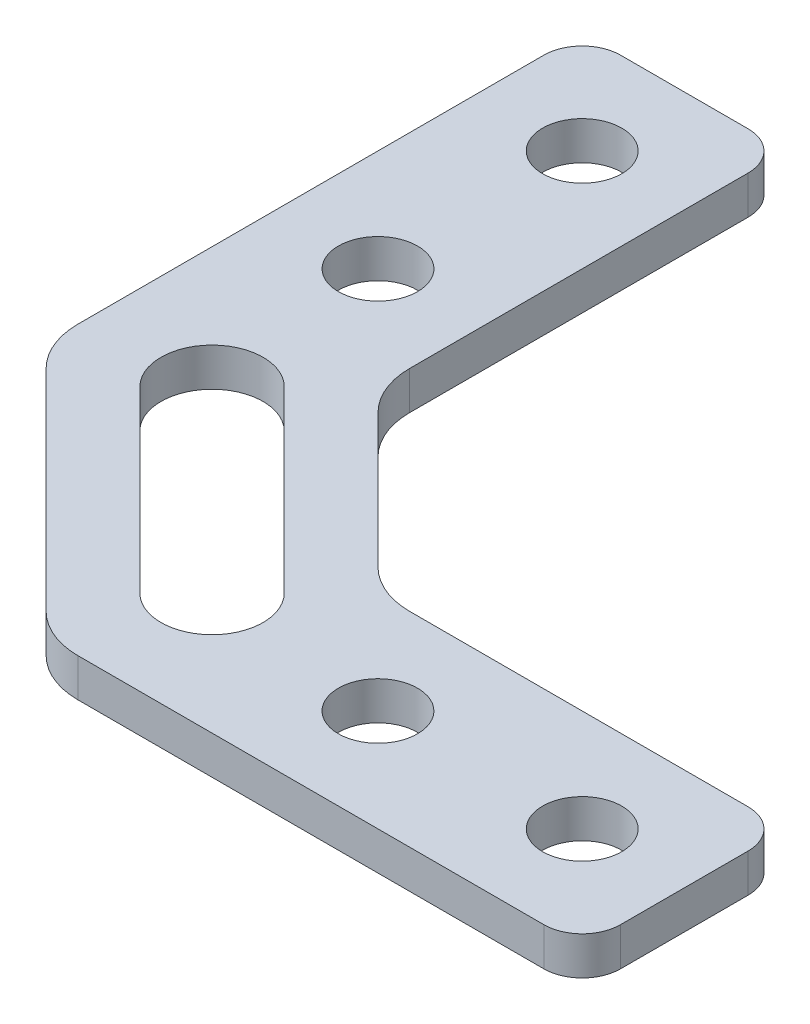
from build123d import *

# Parameters (mm, degrees)
SKETCH_1_R      = 1.55
EXTRUDE_1_DEPTH = 1.5
FILLET_1_R      = 1.5
FILLET_2_R      = 3


with BuildPart() as part:
    # 草图1 → 凸台-拉伸1 (new body)
    with BuildSketch(Plane(origin=(0, 0, 0), x_dir=(1, 0, 0), z_dir=(0, 1, 0))):
        Polygon((27, -4), (27, 4), (11, 4), (4, 11), (4, 27), (-4, 27), (-4, 6), (6, -4), align=None)
        with Locations(Location((15, 0, 0), (0, 0, 270))):
            Circle(SKETCH_1_R, mode=Mode.SUBTRACT)
        with Locations(Location((23, 0, 0), (0, 0, 270))):
            Circle(SKETCH_1_R, mode=Mode.SUBTRACT)
        with Locations(Location((0, 23, 0), (0, 0, 90))):
            Circle(SKETCH_1_R, mode=Mode.SUBTRACT)
        with Locations(Location((0, 15, 0), (0, 0, 90))):
            Circle(SKETCH_1_R, mode=Mode.SUBTRACT)
        with BuildLine():
            Line((2.164213562, 9.164213562), (9.164213562, 2.164213562))
            ThreePointArc((9.164213562, 2.164213562), (9.164213562, -0.664213562), (6.335786438, -0.664213562))
            Line((6.335786438, -0.664213562), (-0.664213562, 6.335786438))
            ThreePointArc((-0.664213562, 6.335786438), (-0.664213562, 9.164213562), (2.164213562, 9.164213562))
        make_face(mode=Mode.SUBTRACT)
    extrude(amount=EXTRUDE_1_DEPTH)

    # 圆角1
    fillet_1_edges = [part.edges().sort_by_distance(p)[0] for p in [
        (-4, 0.75, -27),
        (4, 0.75, -27),
        (27, 0.75, -4),
        (27, 0.75, 4),
    ]]
    fillet(fillet_1_edges, radius=FILLET_1_R)

    # 圆角2
    fillet_2_edges = [part.edges().sort_by_distance(p)[0] for p in [
        (6, 0.75, 4),
        (-4, 0.75, -6),
        (4, 0.75, -11),
        (11, 0.75, -4),
    ]]
    fillet(fillet_2_edges, radius=FILLET_2_R)


solid = part.part
